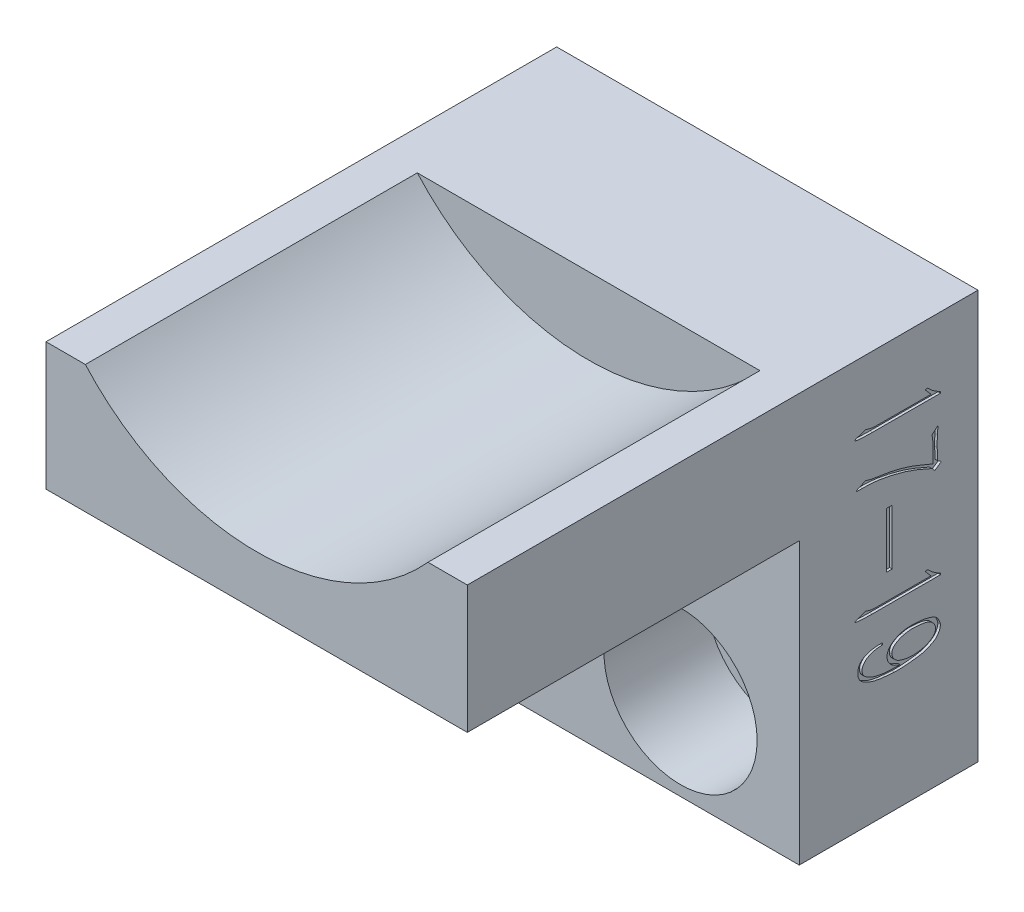
from build123d import *

# Parameters (mm, degrees)
SKETCH1_W                               = 16.5
SKETCH1_H                               = 16
BOSS_EXTRUDE1_DEPTH                     = 20
SKETCH2_W                               = 16.5
SKETCH2_H                               = 11
CUT_EXTRUDE1_DEPTH                      = 13
CBORE_FOR_M3_HEX_HEAD_BOLT1_D           = 3.5
CBORE_FOR_M3_HEX_HEAD_BOLT1_DEPTH       = 7.5
CBORE_FOR_M3_HEX_HEAD_BOLT1_CBORE_D     = 6
CBORE_FOR_M3_HEX_HEAD_BOLT1_CBORE_DEPTH = 4
CBORE_FOR_M3_HEX_HEAD_BOLT1_TIP         = 1.051506083
SKETCH5_R                               = 9
CUT_EXTRUDE2_DEPTH                      = 13
SKETCH7_W                               = 0.217025357
SKETCH7_H                               = 2.164287236
CUT_EXTRUDE4_DEPTH                      = 0.1


with BuildPart() as part:
    # Sketch1 → Boss-Extrude1 (new body)
    with BuildSketch(Plane.XY):
        Rectangle(SKETCH1_W, SKETCH1_H)
    extrude(amount=BOSS_EXTRUDE1_DEPTH)

    # Sketch2 → Cut-Extrude1 (cut)
    with BuildSketch(Plane.XY.offset(20)):
        with Locations((0, -2.5)):
            Rectangle(SKETCH2_W, SKETCH2_H)
    extrude(amount=-CUT_EXTRUDE1_DEPTH, mode=Mode.SUBTRACT)

    # CBORE for M3 Hex Head Bolt1
    with Locations(Plane.XY.offset(7)):
        with Locations((-3.6, -1.4), (3.6, -4.6)):
            CounterBoreHole(CBORE_FOR_M3_HEX_HEAD_BOLT1_D / 2, CBORE_FOR_M3_HEX_HEAD_BOLT1_CBORE_D / 2, CBORE_FOR_M3_HEX_HEAD_BOLT1_CBORE_DEPTH, depth=CBORE_FOR_M3_HEX_HEAD_BOLT1_DEPTH)
            with Locations((0, 0, -(CBORE_FOR_M3_HEX_HEAD_BOLT1_DEPTH + CBORE_FOR_M3_HEX_HEAD_BOLT1_TIP / 2))):  # 118° drill point
                Cone(0, CBORE_FOR_M3_HEX_HEAD_BOLT1_D / 2, CBORE_FOR_M3_HEX_HEAD_BOLT1_TIP, mode=Mode.SUBTRACT)

    # Sketch5 → Cut-Extrude2 (cut)
    with BuildSketch(Plane.XY.offset(20)):
        with Locations((0, 14)):
            Circle(SKETCH5_R)
    extrude(amount=-CUT_EXTRUDE2_DEPTH, mode=Mode.SUBTRACT)

    # Sketch7 → Cut-Extrude4 (cut)
    # profile 1 of 5: a face of its own
    with BuildSketch(Plane(origin=(8.25, 0, 0), x_dir=(0, 0, -1), z_dir=(1, 0, 0))):
        with BuildLine():
            Line((-1.465693586, 5.29501385), (-1.465693586, 5.239825272))
            Line((-1.465693586, 5.239825272), (-4.139356488, 5.245045813))
            add(Edge.make_bspline(
                [(-4.139356488, 5.245045813), (-4.163468776, 5.245640538), (-4.209701405, 5.246780856), (-4.27584832, 5.246873307), (-4.335738169, 5.249049027), (-4.389456903, 5.249221318), (-4.436933695, 5.250841973), (-4.478180463, 5.252703404), (-4.513268625, 5.252908077), (-4.568226249, 5.256073987), (-4.643495265, 5.261942412), (-4.721853245, 5.268689114), (-4.776565212, 5.279102097), (-4.802558686, 5.28527887), (-4.821875074, 5.296177013), (-4.819668022, 5.305960577), (-4.81877264, 5.309929683)],
                knots=[0, 0, 0, 0, 1.451232704, 2.782577199, 3.979589708, 5.056668335, 6.014446553, 6.83767935, 7.540863648, 8.124991547, 10.149851631, 12.075891579, 12.882652565, 13.445716813, 13.775132212, 14, 14, 14, 14], degree=3))
            add(Edge.make_bspline(
                [(-4.81877264, 5.309929683), (-4.818022877, 5.310920212), (-4.81481371, 5.315159919), (-4.808021083, 5.325270446), (-4.789813043, 5.337283837), (-4.773477985, 5.342542549), (-4.763584061, 5.34572768)],
                knots=[0, 0, 0, 0, 0.221265066, 0.947068446, 2.150880552, 4, 4, 4, 4], degree=3))
            Line((-4.763584061, 5.34572768), (-4.6979544, 5.370338802))
            Line((-4.6979544, 5.370338802), (-4.51672704, 5.426273173))
            add(Edge.make_bspline(
                [(-4.51672704, 5.426273173), (-4.49965517, 5.432945867), (-4.469916855, 5.444569355), (-4.431092335, 5.456950167), (-4.405819988, 5.46476276), (-4.385862495, 5.467081494), (-4.366503795, 5.456793354), (-4.337598493, 5.44781085), (-4.300223983, 5.435006911), (-4.25624686, 5.422629449), (-4.208687828, 5.411813147), (-4.157320022, 5.401924122), (-4.099399455, 5.396819202), (-4.044210808, 5.392382326), (-3.990939783, 5.392007471), (-3.939735571, 5.391144357), (-3.879077435, 5.390264259), (-3.835322355, 5.390401747), (-3.811953974, 5.390475176)],
                knots=[0, 0, 0, 0, 1.221104959, 2.127101808, 2.709551176, 2.991566253, 3.431589559, 4.117801824, 5.023798672, 6.056541768, 7.16126461, 8.272176424, 9.537727718, 11.031480746, 11.959016347, 13.085251807, 14.443313417, 16, 16, 16, 16], degree=3))
            Line((-3.811953974, 5.390475176), (-1.838589388, 5.386000426))
            Line((-1.838589388, 5.386000426), (-2.065310036, 5.647773279))
            Line((-2.065310036, 5.647773279), (-1.979544002, 5.667909653))
            add(Edge.make_bspline(
                [(-1.979544002, 5.667909653), (-1.957550615, 5.646639437), (-1.916323103, 5.606767541), (-1.857055366, 5.553361293), (-1.80521643, 5.509711798), (-1.745838776, 5.462938718), (-1.670022189, 5.413037999), (-1.608729863, 5.375150178), (-1.576816535, 5.35542297)],
                knots=[0, 0, 0, 0, 1.077111798, 2.019090495, 2.807993284, 3.46276432, 4.678927073, 6, 6, 6, 6], degree=3))
            Line((-1.576816535, 5.35542297), (-1.465693586, 5.29501385))
        make_face()
    # profile 2 of 5: a face of its own
    with BuildSketch(Plane(origin=(8.25, 0, 0), x_dir=(0, 0, -1), z_dir=(1, 0, 0))):
        with BuildLine():
            add(Edge.make_bspline(
                [(-1.763264436, 2.988280418), (-1.762738695, 3.023829246), (-1.761731363, 3.091941549), (-1.760742565, 3.189145391), (-1.761481816, 3.276903977), (-1.759701309, 3.354713422), (-1.761355597, 3.422826289), (-1.760822313, 3.481249749), (-1.761453841, 3.529989886), (-1.762710473, 3.559310003), (-1.763264436, 3.572235244)],
                knots=[0, 0, 0, 0, 1.461051911, 2.799406174, 3.994695385, 5.067439477, 5.997164994, 6.794024468, 7.468367567, 8, 8, 8, 8], degree=3))
            Line((-1.763264436, 3.572235244), (-1.772959727, 3.813871724))
            add(Edge.make_bspline(
                [(-1.772959727, 3.813871724), (-1.772819112, 3.831637461), (-1.772577195, 3.862202051), (-1.780206187, 3.891742508), (-1.78340081, 3.904112508)],
                knots=[0, 0, 0, 0, 1.16250452, 2, 2, 2, 2], degree=3))
            Line((-1.78340081, 3.904112508), (-1.803537183, 3.954826337))
            add(Edge.make_bspline(
                [(-1.803537183, 3.954826337), (-1.804837016, 3.960809571), (-1.807011698, 3.9708198), (-1.804533951, 3.980688102), (-1.803537183, 3.984658001)],
                knots=[0, 0, 0, 0, 1.19542411, 2, 2, 2, 2], degree=3))
            add(Edge.make_bspline(
                [(-1.803537183, 3.984658001), (-1.801477801, 3.988764216), (-1.796165149, 3.999357143), (-1.779602331, 4.014346978), (-1.757108398, 4.034634495), (-1.73810026, 4.048019924), (-1.727466439, 4.055508204)],
                knots=[0, 0, 0, 0, 0.522008364, 1.346640983, 2.515617707, 4, 4, 4, 4], degree=3))
            Line((-1.727466439, 4.055508204), (-1.606648199, 4.16066482))
            add(Edge.make_bspline(
                [(-1.606648199, 4.16066482), (-1.601213184, 4.164655336), (-1.59289439, 4.170763192), (-1.580114365, 4.178224467), (-1.56995439, 4.171818488), (-1.567765038, 4.164995428), (-1.566375453, 4.16066482)],
                knots=[0, 0, 0, 0, 1.576958087, 2.413680609, 2.993160347, 4, 4, 4, 4], degree=3))
            Line((-1.566375453, 4.16066482), (-1.576816535, 4.059982953))
            Line((-1.576816535, 4.059982953), (-1.586511826, 3.883976135))
            add(Edge.make_bspline(
                [(-1.586511826, 3.883976135), (-1.589478556, 3.842473362), (-1.595106379, 3.763743508), (-1.599545425, 3.651584151), (-1.600888823, 3.55206463), (-1.598200616, 3.489944694), (-1.596952909, 3.461112295)],
                knots=[0, 0, 0, 0, 1.17952993, 2.237542501, 3.181971475, 4, 4, 4, 4], degree=3))
            Line((-1.596952909, 3.461112295), (-1.586511826, 3.012891541))
            Line((-1.586511826, 3.012891541), (-1.435861922, 2.907734924))
            Line((-1.435861922, 2.907734924), (-1.692414234, 2.730982314))
            Line((-1.692414234, 2.730982314), (-1.803537183, 2.851800554))
            add(Edge.make_bspline(
                [(-1.803537183, 2.851800554), (-1.816748896, 2.85718411), (-1.840994884, 2.867063952), (-1.873930325, 2.88188188), (-1.901367104, 2.892503738), (-1.921398273, 2.901212032), (-1.938019316, 2.908501041), (-1.955175569, 2.915952317), (-1.978071453, 2.925838829), (-2.006614665, 2.938372402), (-2.041111117, 2.953108261), (-2.080604853, 2.971391385), (-2.126151171, 2.991413142), (-2.193380602, 3.020498964), (-2.277547953, 3.057618518), (-2.374914651, 3.098634448), (-2.465298794, 3.134361857), (-2.577740505, 3.177081207), (-2.720211331, 3.226203193), (-2.900830634, 3.282209246), (-3.098313108, 3.337562266), (-3.312030778, 3.392066511), (-3.538145944, 3.443879623), (-3.731712007, 3.478065986), (-3.885700273, 3.500465177), (-3.996406754, 3.516256148), (-4.102507129, 3.525914656), (-4.202651915, 3.534577594), (-4.296183911, 3.539554385), (-4.381960762, 3.542646222), (-4.459559818, 3.543676441), (-4.508525049, 3.542305192), (-4.531642872, 3.541657788)],
                knots=[0, 0, 0, 0, 0.452516794, 0.830453727, 1.145288719, 1.385510745, 1.523228126, 1.720999832, 1.978826413, 2.314315288, 2.7098587, 3.168653168, 3.694693257, 4.288008374, 5.492246634, 6.612623083, 7.639124665, 8.574998407, 10.427930525, 12.418278472, 14.572742255, 16.932865428, 19.414160237, 21.929331879, 23.164994651, 24.35049767, 25.475692488, 26.543786625, 27.538913734, 28.446314683, 29.266462724, 30, 30, 30, 30], degree=3))
            Line((-4.531642872, 3.541657788), (-4.747922438, 3.541657788))
            Line((-4.747922438, 3.541657788), (-4.768058811, 3.576709994))
            Line((-4.768058811, 3.576709994), (-4.410824632, 3.73780098))
            add(Edge.make_bspline(
                [(-4.410824632, 3.73780098), (-4.401158805, 3.734713688), (-4.384138184, 3.729277255), (-4.361647566, 3.723467151), (-4.346269061, 3.719521041), (-4.338239421, 3.718136886), (-4.33549968, 3.717664607)],
                knots=[0, 0, 0, 0, 1.560097851, 2.74718673, 3.572535822, 4, 4, 4, 4], degree=3))
            Line((-4.33549968, 3.717664607), (-4.194545067, 3.67739186))
            add(Edge.make_bspline(
                [(-4.194545067, 3.67739186), (-4.16473137, 3.672064156), (-4.101201958, 3.660711457), (-3.999584085, 3.644948045), (-3.886173986, 3.625564669), (-3.764913407, 3.607639927), (-3.645650422, 3.588599514), (-3.537867631, 3.57203804), (-3.446735768, 3.555996998), (-3.366492866, 3.542078017), (-3.286101829, 3.525139859), (-3.194961658, 3.502499306), (-3.08734893, 3.474003552), (-2.96752333, 3.440676405), (-2.842949615, 3.404982795), (-2.722645921, 3.366541369), (-2.609588373, 3.32997016), (-2.537807691, 3.303249791), (-2.503089708, 3.290326017)],
                knots=[0, 0, 0, 0, 0.835892402, 1.781186397, 2.838146302, 4.011381811, 5.164276444, 6.17163188, 7.02104514, 7.718221726, 8.419337669, 9.288042045, 10.30992126, 11.491852482, 12.720884081, 13.886227872, 14.977637142, 16, 16, 16, 16], degree=3))
            Line((-2.503089708, 3.290326017), (-2.054868954, 3.109098658))
            Line((-2.054868954, 3.109098658), (-1.763264436, 2.988280418))
        make_face()
    # profile 3 of 5: a face of its own
    with BuildSketch(Plane(origin=(8.25, 0, 0), x_dir=(0, 0, -1), z_dir=(1, 0, 0))):
        with Locations((-3.467025357, 1.305028766)):
            Rectangle(SKETCH7_W, SKETCH7_H)
    # profile 4 of 5: a face of its own
    with BuildSketch(Plane(origin=(8.25, 0, 0), x_dir=(0, 0, -1), z_dir=(1, 0, 0))):
        with BuildLine():
            Line((-1.465693586, -0.862241636), (-1.465693586, -0.917430215))
            Line((-1.465693586, -0.917430215), (-4.139356488, -0.912209674))
            add(Edge.make_bspline(
                [(-4.139356488, -0.912209674), (-4.163468776, -0.911614949), (-4.209701405, -0.910474631), (-4.27584832, -0.91038218), (-4.335738169, -0.90820646), (-4.389456903, -0.908034169), (-4.436933695, -0.906413514), (-4.478180463, -0.904552083), (-4.513268625, -0.904347409), (-4.568226249, -0.9011815), (-4.643495265, -0.895313075), (-4.721853245, -0.888566373), (-4.776565212, -0.878153389), (-4.802558686, -0.871976617), (-4.821875074, -0.861078473), (-4.819668022, -0.85129491), (-4.81877264, -0.847325804)],
                knots=[0, 0, 0, 0, 1.451232704, 2.782577199, 3.979589708, 5.056668335, 6.014446553, 6.83767935, 7.540863648, 8.124991547, 10.149851631, 12.075891579, 12.882652565, 13.445716813, 13.775132212, 14, 14, 14, 14], degree=3))
            add(Edge.make_bspline(
                [(-4.81877264, -0.847325804), (-4.818022877, -0.846335275), (-4.81481371, -0.842095568), (-4.808021083, -0.831985041), (-4.789813043, -0.819971649), (-4.773477985, -0.814712938), (-4.763584061, -0.811527807)],
                knots=[0, 0, 0, 0, 0.221265066, 0.947068446, 2.150880552, 4, 4, 4, 4], degree=3))
            Line((-4.763584061, -0.811527807), (-4.6979544, -0.786916684))
            Line((-4.6979544, -0.786916684), (-4.51672704, -0.730982314))
            add(Edge.make_bspline(
                [(-4.51672704, -0.730982314), (-4.49965517, -0.72430962), (-4.469916855, -0.712686132), (-4.431092335, -0.70030532), (-4.405819988, -0.692492727), (-4.385862495, -0.690173993), (-4.366503795, -0.700462133), (-4.337598493, -0.709444637), (-4.300223983, -0.722248576), (-4.25624686, -0.734626038), (-4.208687828, -0.74544234), (-4.157320022, -0.755331364), (-4.099399455, -0.760436285), (-4.044210808, -0.764873161), (-3.990939783, -0.765248016), (-3.939735571, -0.76611113), (-3.879077435, -0.766991228), (-3.835322355, -0.76685374), (-3.811953974, -0.766780311)],
                knots=[0, 0, 0, 0, 1.221104959, 2.127101808, 2.709551176, 2.991566253, 3.431589559, 4.117801824, 5.023798672, 6.056541768, 7.16126461, 8.272176424, 9.537727718, 11.031480746, 11.959016347, 13.085251807, 14.443313417, 16, 16, 16, 16], degree=3))
            Line((-3.811953974, -0.766780311), (-1.838589388, -0.771255061))
            Line((-1.838589388, -0.771255061), (-2.065310036, -0.509482208))
            Line((-2.065310036, -0.509482208), (-1.979544002, -0.489345834))
            add(Edge.make_bspline(
                [(-1.979544002, -0.489345834), (-1.957550615, -0.51061605), (-1.916323103, -0.550487946), (-1.857055366, -0.603894194), (-1.80521643, -0.647543689), (-1.745838776, -0.694316768), (-1.670022189, -0.744217488), (-1.608729863, -0.782105309), (-1.576816535, -0.801832517)],
                knots=[0, 0, 0, 0, 1.077111798, 2.019090495, 2.807993284, 3.46276432, 4.678927073, 6, 6, 6, 6], degree=3))
            Line((-1.576816535, -0.801832517), (-1.465693586, -0.862241636))
        make_face()
    # profile 5 of 5: a face of its own
    with BuildSketch(Plane(origin=(8.25, 0, 0), x_dir=(0, 0, -1), z_dir=(1, 0, 0))):
        with BuildLine():
            Line((-3.741103772, -2.086831451), (-3.741103772, -2.157681654))
            add(Edge.make_bspline(
                [(-3.741103772, -2.157681654), (-3.772442627, -2.159452271), (-3.833963595, -2.16292815), (-3.926596106, -2.171986046), (-4.022496713, -2.186180093), (-4.124037447, -2.209446738), (-4.230225728, -2.245404864), (-4.31448286, -2.292203057), (-4.378217207, -2.336149587), (-4.420565322, -2.373383428), (-4.457526939, -2.413582753), (-4.489775969, -2.455406604), (-4.515144698, -2.500674456), (-4.531141629, -2.548792115), (-4.541010571, -2.599015116), (-4.539840027, -2.650341213), (-4.534538471, -2.700183691), (-4.522867317, -2.746017854), (-4.508391405, -2.787750621), (-4.487560232, -2.825799511), (-4.458193098, -2.861735962), (-4.418812221, -2.896875122), (-4.369940871, -2.934237762), (-4.311364039, -2.972967235), (-4.242698446, -3.009904932), (-4.164035823, -3.042524158), (-4.076883952, -3.072305025), (-3.98109831, -3.097863667), (-3.878291411, -3.120139386), (-3.770003862, -3.138470508), (-3.65655177, -3.153510168), (-3.579294788, -3.160778838), (-3.539740038, -3.16450032)],
                knots=[0, 0, 0, 0, 1.252572985, 2.45891248, 3.713291514, 5.118727044, 6.612302482, 8.17054358, 8.946737206, 9.698974805, 10.415081516, 11.123449294, 11.80280777, 12.47422367, 13.139749842, 13.834225331, 14.513511362, 15.13672568, 15.717341908, 16.272390559, 16.858070396, 17.560157575, 18.373746497, 19.312062352, 20.359617366, 21.479952703, 22.706681111, 24.032769727, 25.433856442, 26.903415659, 28.414581869, 30, 30, 30, 30], degree=3))
            Line((-3.539740038, -3.16450032), (-3.24291498, -3.17419561))
            Line((-3.24291498, -3.17419561), (-3.046771788, -3.179416152))
            add(Edge.make_bspline(
                [(-3.046771788, -3.179416152), (-3.066731236, -3.172395067), (-3.104374512, -3.159153386), (-3.156614713, -3.137550579), (-3.20268071, -3.119463528), (-3.254926736, -3.096802419), (-3.313792584, -3.063353358), (-3.382626846, -3.016833856), (-3.446470129, -2.953807341), (-3.495476825, -2.891107832), (-3.529603833, -2.832085753), (-3.547185257, -2.780714165), (-3.557777929, -2.724671783), (-3.559159722, -2.685752091), (-3.559876412, -2.665565736)],
                knots=[0, 0, 0, 0, 0.975313648, 1.839429679, 2.605643894, 3.257344132, 4.462992706, 5.722151988, 7.075833709, 8.579706683, 9.380133085, 10.206640395, 11.069843788, 12, 12, 12, 12], degree=3))
            add(Edge.make_bspline(
                [(-3.559876412, -2.665565736), (-3.559762177, -2.636073672), (-3.559536515, -2.577814633), (-3.534722205, -2.492195102), (-3.490349437, -2.411187449), (-3.435466821, -2.350460411), (-3.382701126, -2.302857989), (-3.33423418, -2.268326991), (-3.280449589, -2.232713423), (-3.19931466, -2.187700581), (-3.090315977, -2.138372998), (-2.974123486, -2.102817233), (-2.875843816, -2.08436818), (-2.795945411, -2.07379557), (-2.709756362, -2.06820721), (-2.587609122, -2.065468937), (-2.433648209, -2.069776043), (-2.311125697, -2.081217767), (-2.251012146, -2.086831451)],
                knots=[0, 0, 0, 0, 0.879679049, 1.737730395, 2.637348044, 3.624206941, 4.172637232, 4.763823156, 5.403988106, 6.104003631, 7.54032698, 8.979426357, 9.729961677, 10.533397673, 11.391675099, 12.315161043, 14.192097489, 16, 16, 16, 16], degree=3))
            add(Edge.make_bspline(
                [(-2.251012146, -2.086831451), (-2.221361227, -2.089849037), (-2.159726547, -2.096121623), (-2.064891051, -2.11527661), (-1.963391113, -2.138688109), (-1.859542906, -2.168955725), (-1.760363455, -2.204332552), (-1.675316787, -2.249477998), (-1.607845348, -2.30358396), (-1.561437551, -2.366450357), (-1.529411228, -2.428691164), (-1.502438196, -2.48413964), (-1.484523763, -2.534181659), (-1.478759532, -2.566038716), (-1.476134669, -2.580545493)],
                knots=[0, 0, 0, 0, 1.076281581, 2.237241691, 3.492213484, 4.839578656, 6.144259871, 7.289828446, 8.304207418, 9.240192607, 10.088260014, 10.83168875, 11.467985033, 12, 12, 12, 12], degree=3))
            add(Edge.make_bspline(
                [(-1.476134669, -2.580545493), (-1.475498671, -2.60446816), (-1.47418836, -2.653754702), (-1.486959168, -2.716052), (-1.504006987, -2.768105078), (-1.525452256, -2.810125763), (-1.550841626, -2.856461278), (-1.584548588, -2.904218887), (-1.62374805, -2.952545747), (-1.671714441, -2.997073015), (-1.726895493, -3.037193935), (-1.809848342, -3.083932852), (-1.918658405, -3.13460802), (-2.031534402, -3.180922817), (-2.130052541, -3.212306837), (-2.218070957, -3.231532769), (-2.319254878, -3.250274846), (-2.429331524, -3.265583443), (-2.537886883, -3.277908767), (-2.634820875, -3.289276078), (-2.715374653, -3.298142967), (-2.802492749, -3.307708839), (-2.906955815, -3.314607151), (-3.032570928, -3.318621788), (-3.154661682, -3.319596414), (-3.232722675, -3.320128466), (-3.268271894, -3.320370765)],
                knots=[0, 0, 0, 0, 0.806662044, 1.661921069, 2.132223286, 2.654585288, 3.252801219, 3.917059286, 4.627088709, 5.35231738, 6.1220317, 6.927642832, 8.566237023, 10.17642927, 11.048081654, 12.056984482, 13.218840013, 14.525927062, 15.811996555, 16.911539304, 17.824569206, 18.551110862, 19.873501701, 21.361558384, 22.79844547, 24, 24, 24, 24], degree=3))
            add(Edge.make_bspline(
                [(-3.268271894, -3.320370765), (-3.327693208, -3.316525545), (-3.441130474, -3.309184893), (-3.604158704, -3.296547767), (-3.754465338, -3.278405667), (-3.896264569, -3.259791349), (-4.032350081, -3.231146399), (-4.166696858, -3.196188887), (-4.301577042, -3.145999569), (-4.411776606, -3.091963536), (-4.496617308, -3.043582466), (-4.549539702, -3.003052456), (-4.594882771, -2.964572086), (-4.636880576, -2.910728014), (-4.672521449, -2.845484346), (-4.699989923, -2.770025842), (-4.709395584, -2.698624649), (-4.70822336, -2.65289362), (-4.707649691, -2.630513531)],
                knots=[0, 0, 0, 0, 1.624314556, 3.1008706, 4.459296012, 5.753938883, 7.000060178, 8.250215639, 9.537556662, 10.917476419, 11.595486364, 12.196294833, 12.734101944, 13.211725603, 14.049516035, 14.752924116, 15.389699498, 16, 16, 16, 16], degree=3))
            add(Edge.make_bspline(
                [(-4.707649691, -2.630513531), (-4.706351039, -2.610576193), (-4.703799653, -2.571406487), (-4.692356615, -2.51377973), (-4.67431649, -2.458928983), (-4.651035041, -2.405990666), (-4.621836527, -2.355740372), (-4.583417531, -2.311132001), (-4.540322372, -2.269184288), (-4.488582869, -2.233720484), (-4.431049834, -2.201790859), (-4.367329407, -2.173095347), (-4.296833272, -2.149924614), (-4.220528254, -2.128767791), (-4.13735829, -2.11154283), (-4.046874381, -2.099380643), (-3.949351322, -2.090113159), (-3.88183202, -2.087948146), (-3.847006179, -2.086831451)],
                knots=[0, 0, 0, 0, 0.842541063, 1.655290544, 2.471486328, 3.274699364, 4.093386327, 4.912812451, 5.751424951, 6.624695527, 7.549987633, 8.526841025, 9.568638607, 10.678378291, 11.867692073, 13.149653009, 14.529816991, 16, 16, 16, 16], degree=3))
            Line((-3.847006179, -2.086831451), (-3.741103772, -2.086831451))
        make_face()
        with BuildLine():
            add(Edge.make_bspline(
                [(-2.523226081, -3.108565949), (-2.477924846, -3.107431147), (-2.3869411, -3.105151991), (-2.249892518, -3.086008656), (-2.112422837, -3.052256793), (-1.998920433, -3.01204748), (-1.911317205, -2.97140726), (-1.850886356, -2.935638809), (-1.796271217, -2.895582402), (-1.747908067, -2.851554593), (-1.707526013, -2.802543799), (-1.679116824, -2.747800917), (-1.6637754, -2.687788188), (-1.66298751, -2.646508741), (-1.66258257, -2.62529299)],
                knots=[0, 0, 0, 0, 1.505084237, 3.022835914, 4.587793371, 6.202784538, 7.015839827, 7.793714509, 8.5323415, 9.263164892, 9.962488781, 10.631279674, 11.296540223, 12, 12, 12, 12], degree=3))
            add(Edge.make_bspline(
                [(-1.66258257, -2.62529299), (-1.664285477, -2.606246759), (-1.667723589, -2.56779307), (-1.687549268, -2.51205942), (-1.71717461, -2.458109459), (-1.757218081, -2.407972608), (-1.803653146, -2.362277617), (-1.854625056, -2.322774435), (-1.910066488, -2.292095888), (-1.969958893, -2.269792564), (-2.033743505, -2.252133734), (-2.102796638, -2.237423503), (-2.177386038, -2.224515177), (-2.282700197, -2.212728249), (-2.412875385, -2.200509634), (-2.541012862, -2.192064581), (-2.641697531, -2.19247043), (-2.719751929, -2.199415051), (-2.801694531, -2.212943062), (-2.85716625, -2.226194743), (-2.885680801, -2.233006606)],
                knots=[0, 0, 0, 0, 0.723074811, 1.459863333, 2.223981372, 3.050472336, 3.884251909, 4.691738036, 5.489747144, 6.278052458, 7.111191484, 7.999281961, 8.956099049, 9.982199247, 12.019015077, 13.91785247, 14.851750992, 15.836432574, 16.887844892, 18, 18, 18, 18], degree=3))
            add(Edge.make_bspline(
                [(-2.885680801, -2.233006606), (-2.909673038, -2.238260671), (-2.957490747, -2.248732282), (-3.026698233, -2.272641267), (-3.094027162, -2.299816581), (-3.157147151, -2.332091272), (-3.213754581, -2.367590404), (-3.263305124, -2.403345185), (-3.301459261, -2.442810777), (-3.33170206, -2.482528032), (-3.352014782, -2.524854115), (-3.365789864, -2.568487078), (-3.372011933, -2.614469892), (-3.369981354, -2.645425578), (-3.368953761, -2.661090987)],
                knots=[0, 0, 0, 0, 1.249598274, 2.490510859, 3.722286335, 4.945118518, 6.093691385, 7.124089869, 8.046071331, 8.879029982, 9.654610032, 10.423342017, 11.202117798, 12, 12, 12, 12], degree=3))
            add(Edge.make_bspline(
                [(-3.368953761, -2.661090987), (-3.367406511, -2.679855364), (-3.364362317, -2.716774044), (-3.347912777, -2.769624218), (-3.323906674, -2.818808169), (-3.291524651, -2.863378173), (-3.253618309, -2.902814684), (-3.213332277, -2.938254683), (-3.170393972, -2.968208237), (-3.124481076, -2.994224686), (-3.073751604, -3.016847406), (-3.016648508, -3.036086558), (-2.953961462, -3.057156026), (-2.883564426, -3.074381132), (-2.805713031, -3.091016694), (-2.719042206, -3.100329509), (-2.624030222, -3.107540237), (-2.5577984, -3.108214166), (-2.523226081, -3.108565949)],
                knots=[0, 0, 0, 0, 0.858414698, 1.68892027, 2.512241944, 3.35110229, 4.195180626, 5.008719287, 5.800048783, 6.583753001, 7.417982137, 8.334529499, 9.337205384, 10.439689195, 11.64539845, 12.973188474, 14.420036011, 16, 16, 16, 16], degree=3))
        make_face(mode=Mode.SUBTRACT)
    extrude(amount=-CUT_EXTRUDE4_DEPTH, mode=Mode.SUBTRACT)


solid = part.part
